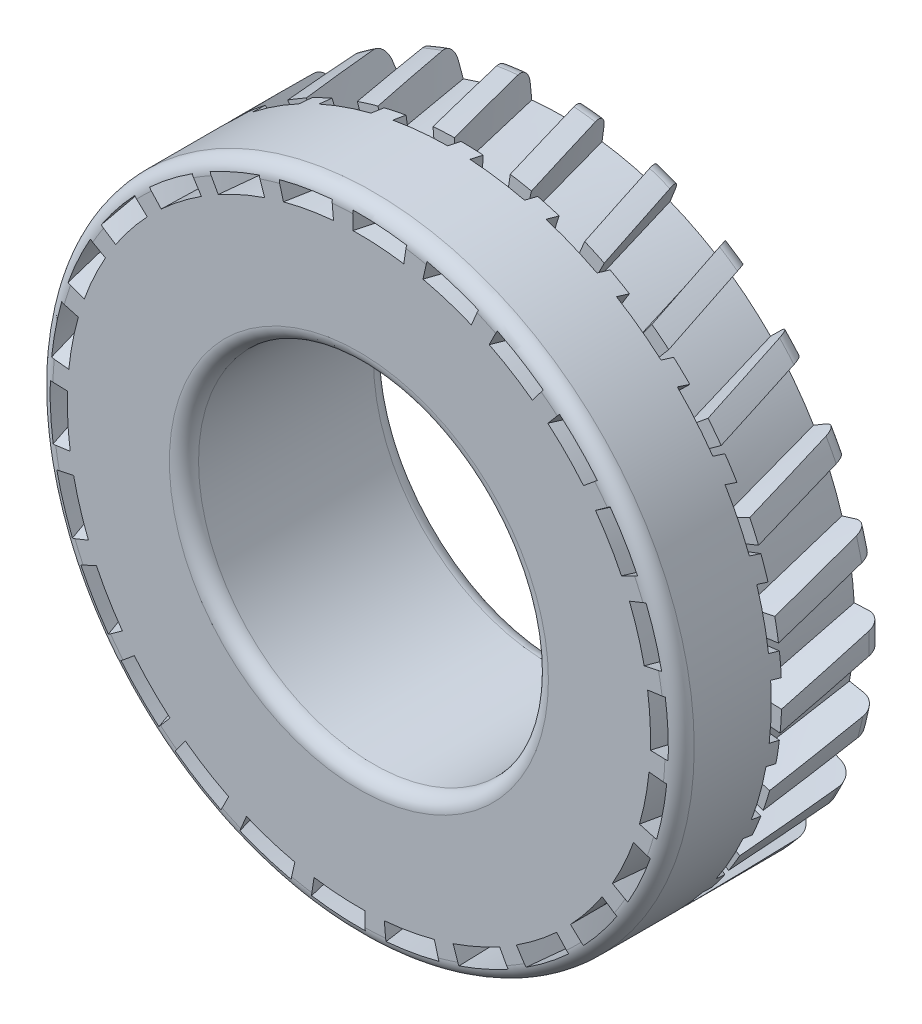
from build123d import *

# Parameters (mm, degrees)
SKETCH_1_R               = 220
SKETCH_1_R_2             = 120
EXTRUDE_1_DEPTH          = 70
FILLET_5_R               = 10
PATTERN_CIRCULAR_1_COUNT = 26
PATTERN_CIRCULAR_2_COUNT = 26


with BuildPart() as part:
    # 草图1 → 凸台-拉伸1 (new, symmetric)
    with BuildSketch(Plane.XY):
        Circle(SKETCH_1_R)
        Circle(SKETCH_1_R_2, mode=Mode.SUBTRACT)
    extrude(amount=EXTRUDE_1_DEPTH, both=True)

    # 圆角5
    fillet_5_edges = [part.edges().sort_by_distance(p)[0] for p in [
        (-220, 0, -70),
        (-220, 0, 70),
        (-120, 0, -70),
        (-120, 0, 70),
    ]]
    fillet(fillet_5_edges, radius=FILLET_5_R)

    # 草图5 for 切除-放样3 → 切除-放样3 section 0
    with BuildSketch(Plane.XY):
        with BuildLine():
            Line((-37.857421254, 217.733359079), (-34.210798078, 197.052331361))
            # circular arc as an exact rational Bezier (weights 1, cos(half-angle), 1)
            Bezier((-34.210798078, 197.052331361), (-17.232387459, 200), (0, 200), weights=[1, 0.996308601, 1])
            Line((0, 200), (0, 221))
            Bezier((0, 221), (-19.069646572, 221), (-37.857421254, 217.733359079), weights=[1, 0.996297852, 1])
        make_face()
    # 草图6 for 切除-放样3 → 切除-放样3 section 1
    with BuildSketch(Plane.XY.offset(70)):
        with BuildLine():
            Line((-17.43114855, 199.238939618), (-18.477017463, 211.193275995))
            Bezier((-18.477017463, 211.193275995), (-36.954034925, 209.576746432), (-54.869637562, 204.776275173), weights=[1, 0.996194698, 1])
            Line((-54.869637562, 204.776275173), (-51.763809021, 193.185165258))
            Bezier((-51.763809021, 193.185165258), (-34.862297099, 197.713911728), (-17.43114855, 199.238939618), weights=[1, 0.996194698, 1])
        make_face()
    loft_3 = loft(mode=Mode.SUBTRACT)

    # 阵列(圆周)1: 切除-放样3 ×26 about axis
    pattern_circular_1_axis = Axis((0, 0, 70), (0, 0, 1))
    for i in range(1, PATTERN_CIRCULAR_1_COUNT):
        add(loft_3.rotate(pattern_circular_1_axis, i * 360 / PATTERN_CIRCULAR_1_COUNT), mode=Mode.SUBTRACT)

    # 草图8 for 切除-放样4 → 切除-放样4 section 0
    with BuildSketch(Plane(origin=(0, 0, -70), x_dir=(-1, 0, 0), z_dir=(0, 0, -1))):
        with BuildLine():
            Line((38.376247264, 217.642513416), (34.729635533, 196.961550602))
            Bezier((34.729635533, 196.961550602), (51.961538362, 193.923101205), (68.404028665, 187.938524157), weights=[1, 0.996194698, 1])
            Line((68.404028665, 187.938524157), (75.586451675, 207.672069194))
            Bezier((75.586451675, 207.672069194), (57.41749989, 214.285026831), (38.376247264, 217.642513416), weights=[1, 0.996194698, 1])
        make_face()
    # 草图7 for 切除-放样4 → 切除-放样4 section 1
    with BuildSketch(Plane.XY):
        with BuildLine():
            Line((-17.43114855, 199.238939618), (-19.261419147, 220.159028278))
            Bezier((-19.261419147, 220.159028278), (-38.522838294, 218.473872459), (-57.199008968, 213.46960761), weights=[1, 0.996194698, 1])
            Line((-57.199008968, 213.46960761), (-51.763809021, 193.185165258))
            Bezier((-51.763809021, 193.185165258), (-34.862297099, 197.713911728), (-17.43114855, 199.238939618), weights=[1, 0.996194698, 1])
        make_face()
    loft_4 = loft(mode=Mode.SUBTRACT)

    # 阵列(圆周)2: 切除-放样4 ×26 about axis
    pattern_circular_2_axis = Axis((0, 0, 70), (0, 0, 1))
    for i in range(1, PATTERN_CIRCULAR_2_COUNT):
        add(loft_4.rotate(pattern_circular_2_axis, i * 360 / PATTERN_CIRCULAR_2_COUNT), mode=Mode.SUBTRACT)


solid = part.part
